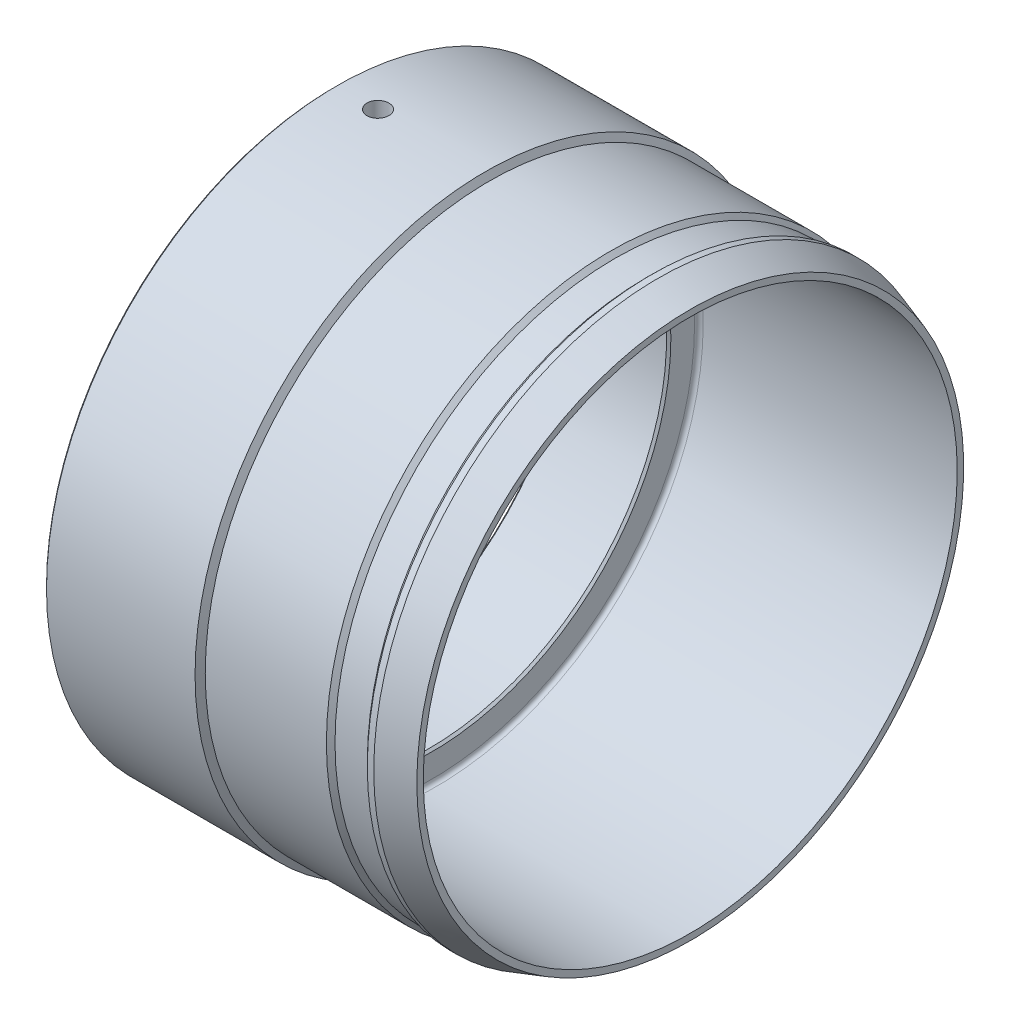
from build123d import *

# Parameters (mm, degrees)
FILLET1_R          = 2
CHAMFER1_SIZE      = 1
M12_TAPPED_HOLE1_D = 10.2


with BuildPart() as part:
    # Sketch1 → Revolve1 (revolve)
    with BuildSketch(Plane.XY, mode=Mode.PRIVATE) as revolve1_sk:
        Polygon((0, 110), (45, 110), (45, 124), (165, 124), (165, 127), (150, 132), (147, 132), (145, 130), (130, 130), (128, 132), (71.732050808, 132), (70, 135), (0, 135), align=None)
    revolve(revolve1_sk.sketch.rotate(Axis((0, 0, 0), (1, 0, 0)), 90), axis=Axis((0, 0, 0), (1, 0, 0)))

    # Fillet1
    fillet1_edges = [part.edges().sort_by_distance(p)[0] for p in [
        (45, 0, -124),
    ]]
    fillet(fillet1_edges, radius=FILLET1_R)

    # Chamfer1
    chamfer1_edges = [part.edges().sort_by_distance(p)[0] for p in [
        (45, 0, -110),
        (0, 0, -110),
        (0, 0, -135),
    ]]
    chamfer(chamfer1_edges, length=CHAMFER1_SIZE)

    # M12 Tapped Hole1 (through all)
    with Locations(Plane(origin=(20, 135, 0), x_dir=(0, 0, 1), z_dir=(0, 1, 0))):
        with Locations((0, 0)):
            Hole(M12_TAPPED_HOLE1_D / 2)


solid = part.part
